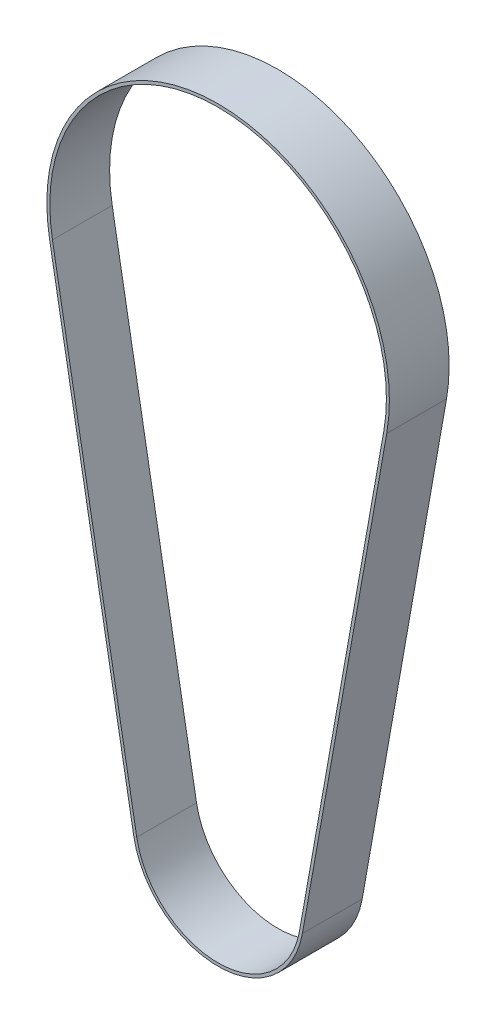
from build123d import *

# Parameters (mm, degrees)
BOSS_EXTRUDE1_DEPTH = 5


with BuildPart() as part:
    # Sketch1 → Boss-Extrude1 (new, symmetric)
    with BuildSketch(Plane.XY):
        with BuildLine():
            Line((-28.209436762, 76.994984756), (-14.104718381, -2.502507622))
            ThreePointArc((-14.104718381, -2.502507622), (0, -14.325), (14.104718381, -2.502507622))
            Line((14.104718381, -2.502507622), (28.209436762, 76.994984756))
            ThreePointArc((28.209436762, 76.994984756), (0, 110.65), (-28.209436762, 76.994984756))
        make_face()
        with BuildLine():
            Line((-27.717125474, 77.082332317), (-13.612407094, -2.415160061))
            ThreePointArc((-13.612407094, -2.415160061), (0, -13.825), (13.612407094, -2.415160061))
            Line((13.612407094, -2.415160061), (27.717125474, 77.082332317))
            ThreePointArc((27.717125474, 77.082332317), (0, 110.15), (-27.717125474, 77.082332317))
        make_face(mode=Mode.SUBTRACT)
    extrude(amount=BOSS_EXTRUDE1_DEPTH, both=True)


solid = part.part
